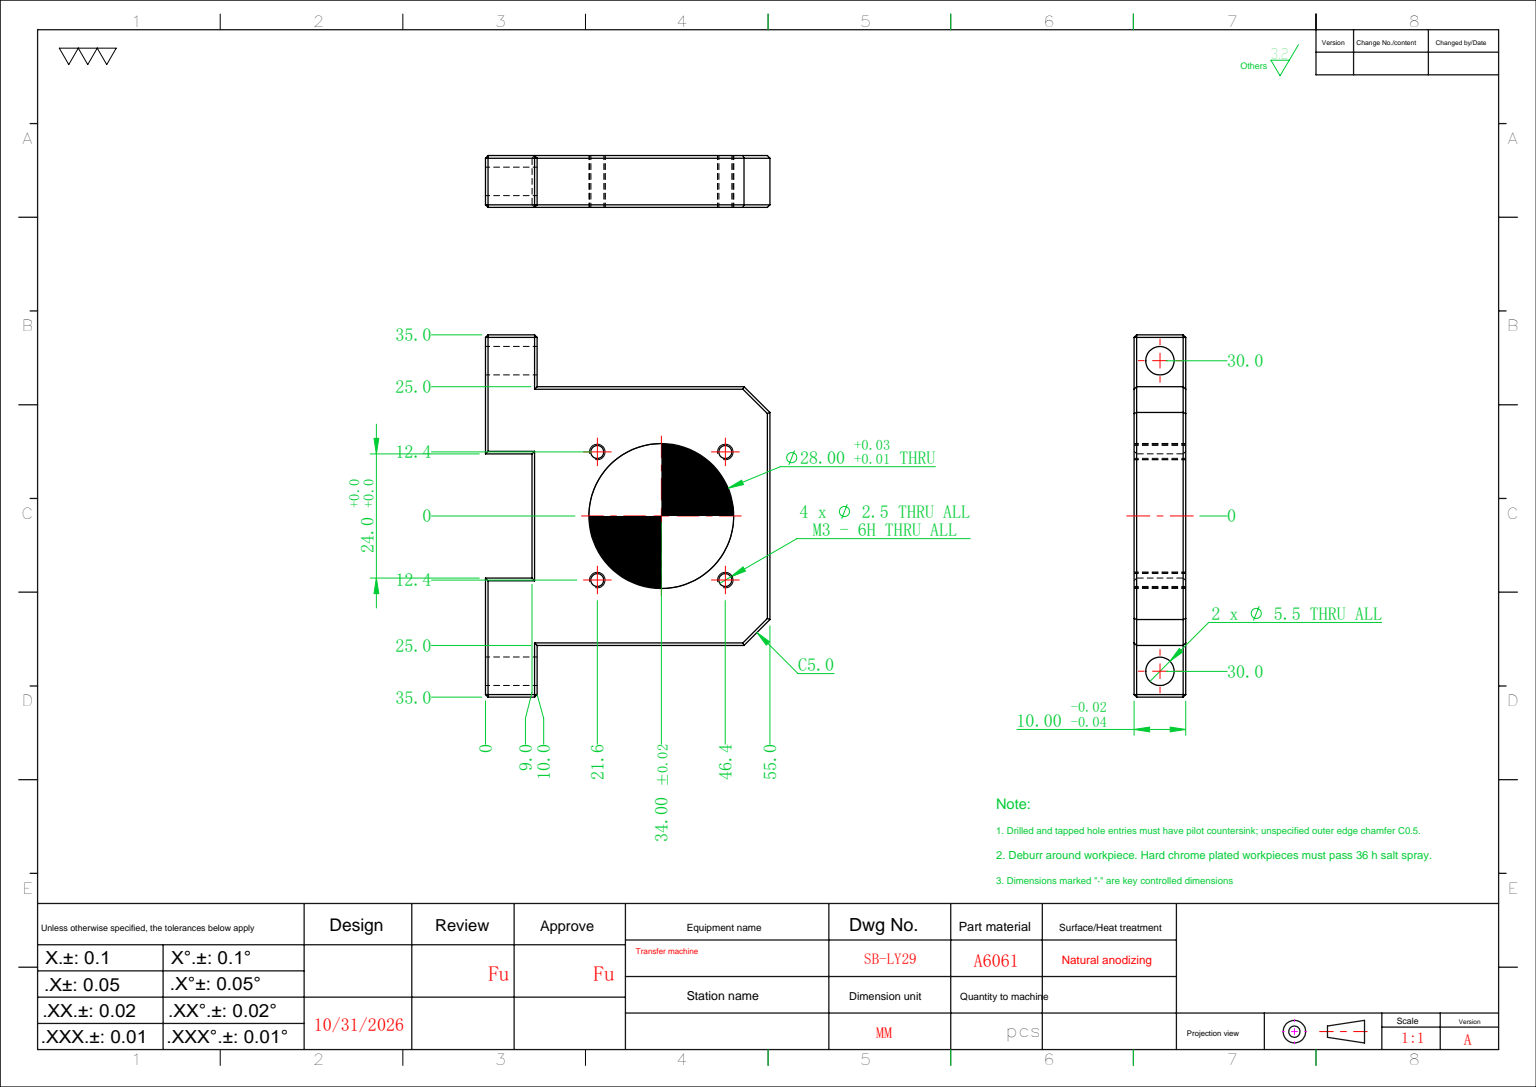
from build123d import *

# Parameters (mm, degrees)
SKETCH_1_W              = 70
SKETCH_1_H              = 55
EXTRUDE_1_DEPTH         = 10
SKETCH_2_W              = 10
SKETCH_2_H              = 45
CUT_EXTRUDE_1_DEPTH     = 46.620718977
SKETCH_3_R              = 14
CUT_EXTRUDE_2_DEPTH     = 46.620718977
HOLE_WIZARD_M3_1_D      = 2.5
HOLE_WIZARD_5_5_5_5_1_D = 5.5
CHAMFER_1_SIZE          = 5
SKETCH_12_W             = 24
SKETCH_12_H             = 9
CUT_EXTRUDE_3_DEPTH     = 46.620718977
CHAMFER_2_SIZE          = 0.5


with BuildPart() as part:
    # 草图1 → 凸台-拉伸1 (new body)
    with BuildSketch(Plane.XY):
        Rectangle(SKETCH_1_W, SKETCH_1_H)
    extrude(amount=EXTRUDE_1_DEPTH)

    # 草图2 → 切除-拉伸1 (cut, through all)
    with BuildSketch(Plane.XY.offset(10)):
        with Locations((-30, -5)):
            Rectangle(SKETCH_2_W, SKETCH_2_H)
        with Locations((30, -5)):
            Rectangle(SKETCH_2_W, SKETCH_2_H)
    extrude(amount=-CUT_EXTRUDE_1_DEPTH, mode=Mode.SUBTRACT)

    # 草图3 → 切除-拉伸2 (cut, through all)
    with BuildSketch(Plane(origin=(0, 0, 0), x_dir=(-1, 0, 0), z_dir=(0, 0, -1))):
        with Locations((0, -6.5)):
            Circle(SKETCH_3_R)
    extrude(amount=-CUT_EXTRUDE_2_DEPTH, mode=Mode.SUBTRACT)

    # M3 螺纹孔1 (through all)
    with Locations(Plane.XY.offset(10)):
        with Locations((12.375, -18.875), (-12.375, -18.875), (-12.375, 5.875), (12.375, 5.875)):
            Hole(HOLE_WIZARD_M3_1_D / 2)

    # Ø5.5 (5.5) 直径孔1 (through all)
    with Locations(Plane(origin=(0, 17.5, 0), x_dir=(-1, 0, 0), z_dir=(0, -1, 0))):
        with Locations((-30, -5), (30, -5)):
            Hole(HOLE_WIZARD_5_5_5_5_1_D / 2)

    # 倒角1
    chamfer_1_edges = [part.edges().sort_by_distance(p)[0] for p in [
        (-25, -27.5, 5),
        (25, -27.5, 5),
    ]]
    chamfer(chamfer_1_edges, length=CHAMFER_1_SIZE)

    # 草图12 → 切除-拉伸3 (cut, through all)
    with BuildSketch(Plane.XY.offset(10)):
        with Locations((0, 23)):
            Rectangle(SKETCH_12_W, SKETCH_12_H)
    extrude(amount=-CUT_EXTRUDE_3_DEPTH, mode=Mode.SUBTRACT)

    # 倒角2
    chamfer_2_edges = [part.edges().sort_by_distance(p)[0] for p in [
        (-35, 22.5, 10),
        (0, 18.5, 10),
        (12, 23, 10),
        (-30, 17.5, 0),
        (-35, 17.5, 5),
        (-30, 17.5, 10),
        (35, 22.5, 0),
        (35, 22.5, 10),
        (25, -2.5, 0),
        (30, 17.5, 0),
        (35, 17.5, 5),
        (30, 17.5, 10),
        (25, -2.5, 10),
        (-35, 22.5, 0),
        (23.5, 27.5, 0),
        (23.5, 27.5, 10),
        (-35, 27.5, 5),
        (35, 27.5, 5),
        (-25, -2.5, 10),
        (-25, -2.5, 0),
        (0, -27.5, 10),
        (22.5, -25, 10),
        (-22.5, -25, 10),
        (0, -27.5, 0),
        (22.5, -25, 0),
        (-22.5, -25, 0),
        (-23.5, 27.5, 0),
        (-23.5, 27.5, 10),
        (-12, 23, 0),
        (12, 23, 0),
        (0, 18.5, 0),
        (-12, 23, 10),
    ]]
    chamfer(chamfer_2_edges, length=CHAMFER_2_SIZE)


solid = part.part
